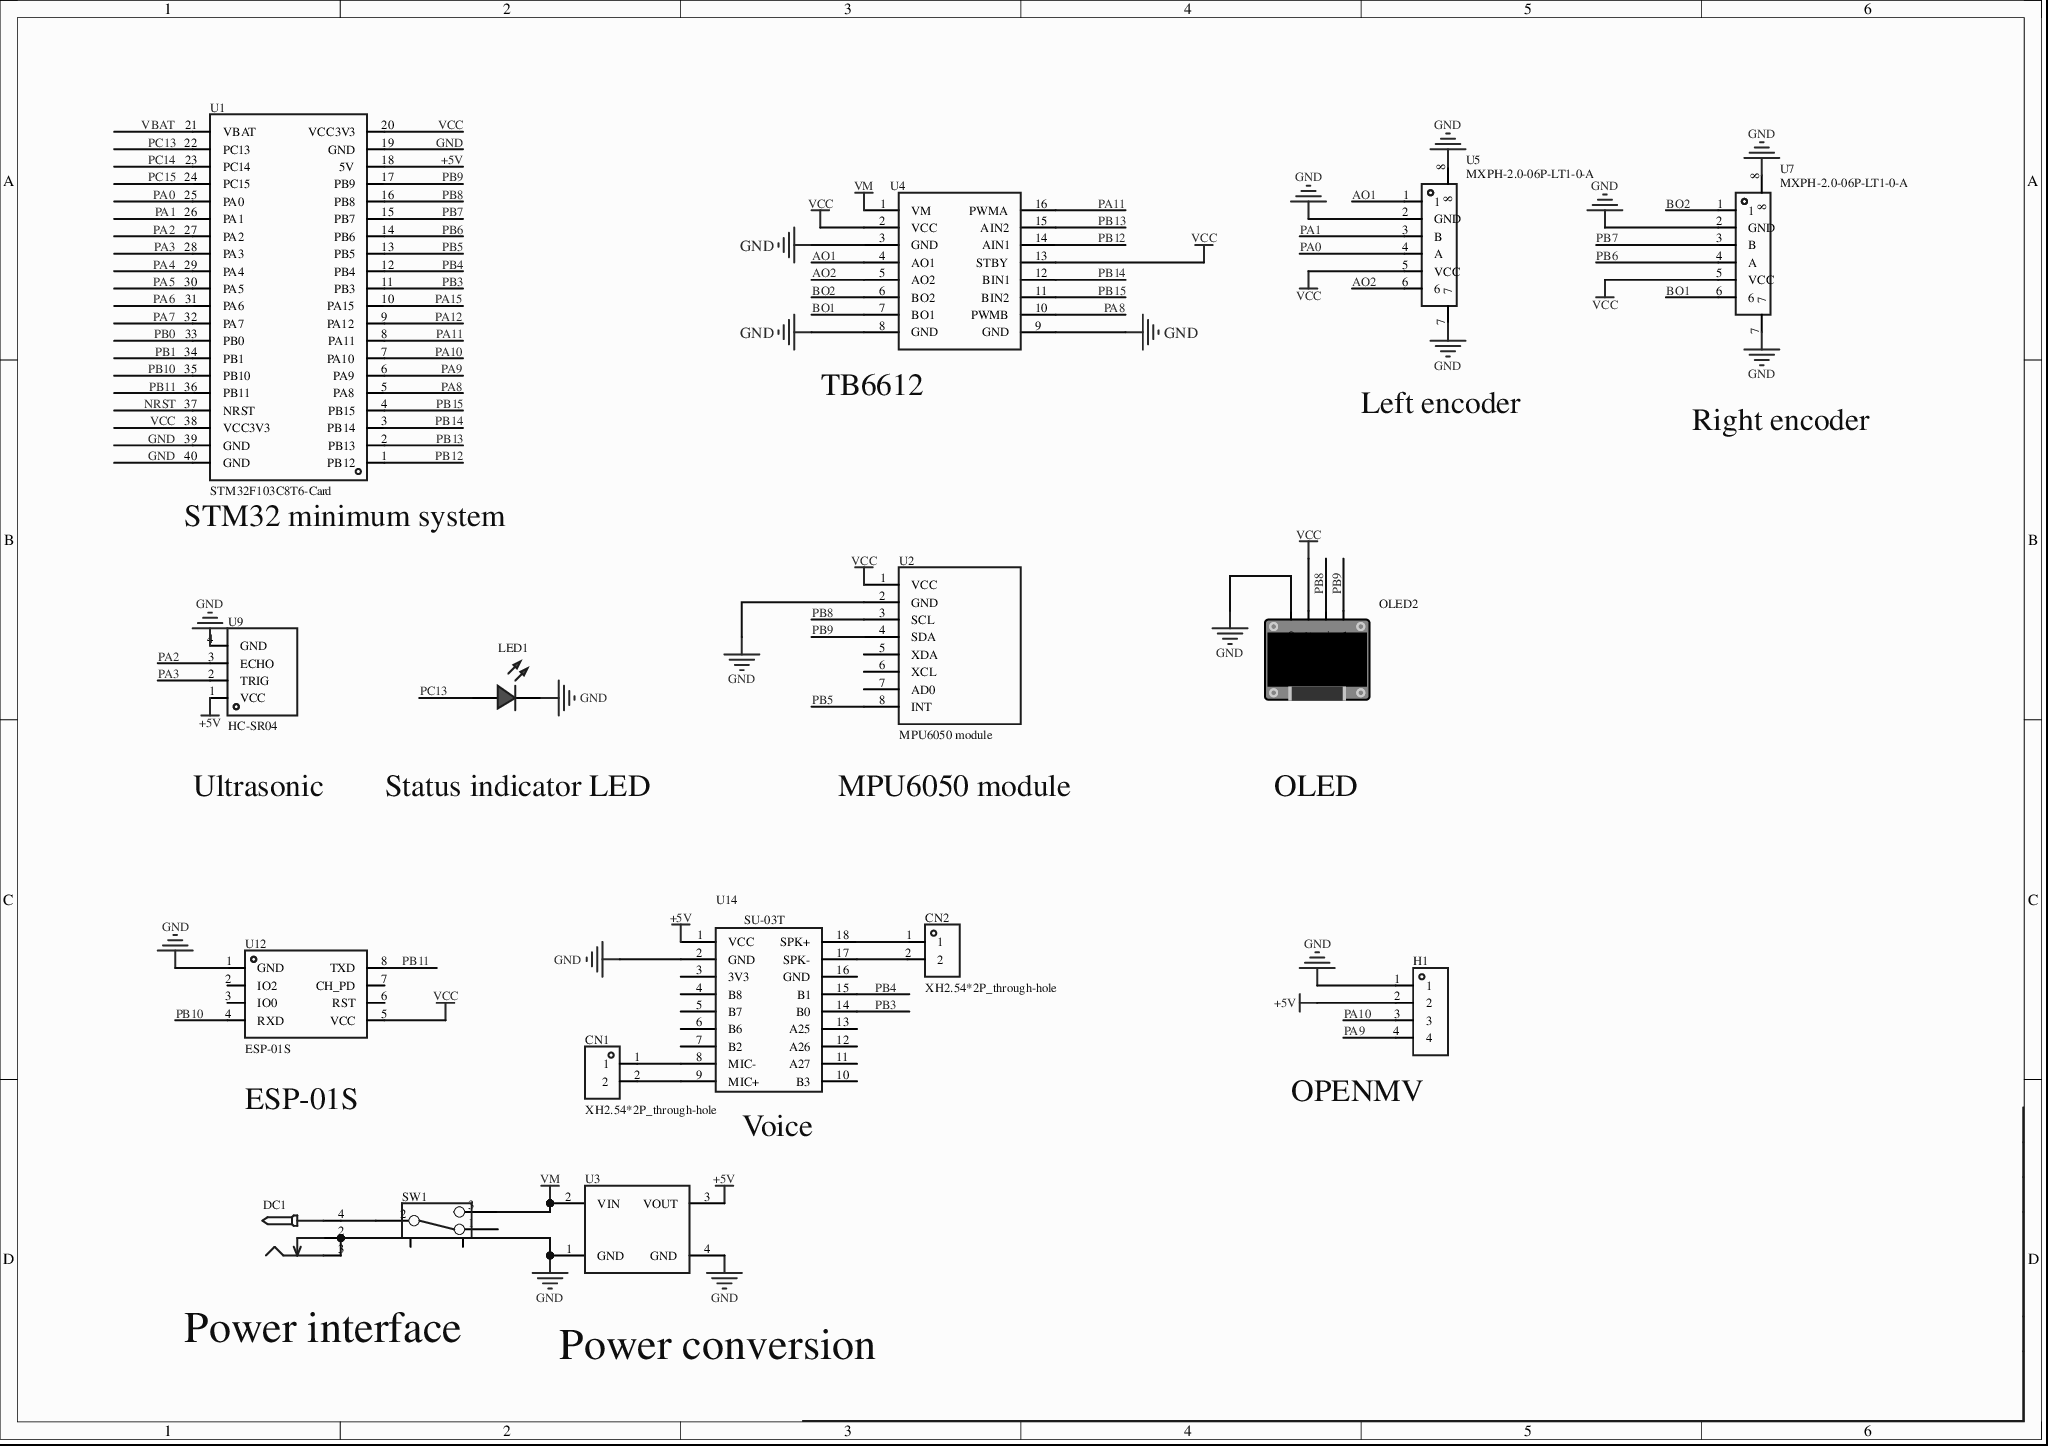
[diagram p0: MISC61229-3.schdoc]
# Altium project MISC61229-2.PrjPcb
1 sheet, 16 parts. Net scope: global (net labels, ports and power ports of the same name join across sheets).
Board file: MISC61229.pcbdoc

## Sheet MISC61229-3.schdoc
size 297 x 209 mm; Version: V1.0; @Project Name: MISC61229; @Page Count: 1; @Update Date: 2026-05-19; @Create Date: 2026-05-19; @Schematic Name: MISC61229; @Page No: 1; @Create Time: 23:22:16; @Update Time: 17:32:40; @Board Name: MISC61229

### Parts
CN1  XH2.54*2P_through-hole  [CONN-TH_2P-P2.50-XH2.54-2P]
CN2  XH2.54*2P_through-hole  [CONN-TH_2P-P2.50-XH2.54-2P]
DC1  (no value)  [DC-2.0]
H1  (no value)  [HDR-TH_4P-P2.54-V-M]
LED1  (no value)  [LED_TH-3mm]
OLED2  (no value)  [0.96OLED_4P]
SW1  (no value)  [拨动开关]
U1  STM32F103C8T6-Card  [CONN-TH_L53.3-W22.9_STM32F103C8T6-CARD]
U2  MPU6050 module  [MPU6050]
U3  (no value)  [MP1584主控]
U4  (no value)  [tb6612]
U5  MXPH-2.0-06P-LT1-0-A  [CONN-SMD_6P-P2.00_MXPH-2.0-6P-LT1-0-A]
U7  MXPH-2.0-06P-LT1-0-A  [CONN-SMD_6P-P2.00_MXPH-2.0-6P-LT1-0-A]
U9  HC-SR04  [TH_HC-SR04V]
U12  ESP-01S  [WIFIM-TH_ESP-01S]
U14  (no value)  [SU-03T]

### Nets
+5V: H1.2 U1.18(5V) U3.3(VOUT) U9.1(VCC) U14.1(VCC)
GND: DC1.2 DC1.3 H1.1 LED1.2(A) OLED2.1(GND) U1.19(GND) U1.39(GND) U1.40(GND) U2.2(GND) U3.1(GND) U3.4(GND) U4.3(GND) U4.8(GND) U4.9(GND) U5.2(GND) U5.7 U5.8 U7.2(GND) U7.7 U7.8 U9.4(GND) U12.1(GND) U14.2(GND)
VCC: OLED2.2(VCC) U1.20(VCC3V3) U1.38(VCC3V3) U2.1(VCC) U4.2(VCC) U4.13(STBY) U5.5(VCC) U7.5(VCC) U12.5(VCC)
VM: SW1.3 U3.2(VIN) U4.1(VM)
AO1: U4.4(AO1) U5.1
AO2: U4.5(AO2) U5.6
BO1: U4.7(BO1) U7.6
BO2: U4.6(BO2) U7.1
NRST: U1.37(NRST)
PA0: U1.25(PA0) U5.4(A)
PA1: U1.26(PA1) U5.3(B)
PA2: U1.27(PA2) U9.3(ECHO)
PA3: U1.28(PA3) U9.2(TRIG)
PA4: U1.29(PA4)
PA5: U1.30(PA5)
PA6: U1.31(PA6)
PA7: U1.32(PA7)
PA8: U1.5(PA8) U4.10(PWMB)
PA9: H1.4 U1.6(PA9)
PA10: H1.3 U1.7(PA10)
PA11: U1.8(PA11) U4.16(PWMA)
PA12: U1.9(PA12)
PA15: U1.10(PA15)
PB0: U1.33(PB0)
PB1: U1.34(PB1)
PB3: U1.11(PB3) U14.14(B0)
PB4: U1.12(PB4) U14.15(B1)
PB5: U1.13(PB5) U2.8(INT)
PB6: U1.14(PB6) U7.4(A)
PB7: U1.15(PB7) U7.3(B)
PB8: OLED2.3(SCL) U1.16(PB8) U2.3(SCL)
PB9: OLED2.4(SDA) U1.17(PB9) U2.4(SDA)
PB10: U1.35(PB10) U12.4(RXD)
PB11: U1.36(PB11) U12.8(TXD)
PB12: U1.1(PB12) U4.14(AIN1)
PB13: U1.2(PB13) U4.15(AIN2)
PB14: U1.3(PB14) U4.12(BIN1)
PB15: U1.4(PB15) U4.11(BIN2)
PC13: LED1.1(C) U1.22(PC13)
PC14: U1.23(PC14)
PC15: U1.24(PC15)
VBAT: U1.21(VBAT)
NetCN1_1: CN1.1 U14.8(MIC-)
NetCN1_2: CN1.2 U14.9(MIC+)
NetCN2_1: CN2.1 U14.18(SPK+)
NetCN2_2: CN2.2 U14.17(SPK-)
NetDC1_4: DC1.4 SW1.2

Not connected (* = marked no-connect by the designer): SW1 1 4 5; U2 5(XDA) 6(XCL) 7(AD0); U12 2(IO2)* 3(IO0)* 6(RST)* 7(CH_PD)*; U14 3(3V3) 4(B8) 5(B7) 6(B6) 7(B2) 10(B3) 11(A27) 12(A26) 13(A25) 16(GND)

### Notes on the sheet
- (near U4) TB6612
- Left encoder
- Right encoder
- (near U1) STM32 minimum system
- Ultrasonic
- Status indicator LED
- (near U2) MPU6050 module
- OLED
- (near U12) ESP-01S
- (near H1) OPENMV
- (near U14) Voice
- Power interface
- (near U3) Power conversion

### Library data of the parts
CN1 CN2 = XH2.54*2P_直插: AddInBom: yes; ModelId: 325c595e30db4df8abe76612dd40b0fa0819f05c4eef4c71ace90d822a990e87; ModelTransform: 295.275,228.346,0,180,0,0,-0.002,-20.079,-137.795; Symbol: XH2.54*2P_through-hole; Device: XH2.54*2P_through-hole; LCSC Part Name: XH2.54*2P_直插; SupplierPart: C9900008615; ManufacturerPart: XH2.54*2P_直插; Supplier Footprint: XH2.54_2P; JLCPCB Part Class: Extended Part; Supplier: LCSC; ConvertToPcb: yes; FootprintName: CONN-TH_2P-P2.50-XH2.54-2P; ModelName: CONN-TH_2P-P2.50-XH2.54-2P
DC1 = DC-005_2.0: Symbol: DC power connector; ConvertToPcb: yes; ModelId: f5f20b8a2308479b936ba3c2698865bb0819f05c4eef4c71ace90d822a990e87; ModelName: DC-IN-TH_DC-5520-1; ModelTransform: 372.05,551.18,582.68,90,0,0,137.8,0,-149.61; Device: DC-005_2.0; AddInBom: yes; Supplier Footprint: 插件; FootprintName: DC-2.0
H1 = HDR-M_2.54_1x4P: Symbol: PZ254V-11-04P; ConvertToPcb: yes; ModelId: 112f4d05e8d64e99ab9a333894bea4f90819f05c4eef4c71ace90d822a990e87; ModelName: HDR-TH_4P-P2.54-M-LI-1X4P; ModelTransform: 399.999,104.7242,0,0,0,0,0,0,-118.11; Device: HDR-M_2.54_1x4P; AddInBom: yes; SupplierPart: C492403; Supplier Footprint: 插件; FootprintName: HDR-TH_4P-P2.54-V-M
LED1 = LED_TH-R_3mm: ConvertToPcb: yes; ModelId: a497c992633541038a38947cdc58012f0819f05c4eef4c71ace90d822a990e87; ModelName: LED-TH-3mm_R; ModelTransform: 141.274,153.327,0,0,0,0,-5.984,0,-137.795; Symbol: LED_TH-R; Device: LED_TH-R_3mm; AddInBom: yes; FootprintName: LED_TH-3mm; Supplier Footprint: 插件
OLED2 = 0.96OLED模块_4P: Symbol: 0.96OLED module_4P; 3D Model: 79c000fdb68d45a296c2e9bedf4f9055; 3D Model Transform: 1393.69792,1318.895,0,0,0,0,0,-560.079,-137.795; ConvertToPcb: yes; Device: 0.96OLED module_4P; Supplier Footprint: 插件; AddInBom: yes; FootprintName: 0.96OLED_4P; ModelName: 0.96OLED_4P
SW1 = 拨动开关_正: Symbol: Toggle switch; Device: Toggle switch_positive; ConvertToPcb: yes; ModelId: 4321fe59a4074cbfb4989553f297c68f0819f05c4eef4c71ace90d822a990e87; ModelName: SW-TH_SS-12D02-VG4; ModelTransform: 370.09,208.7,472.35,0,0,0,0,0,-110; AddInBom: yes; Supplier Footprint: 插件; FootprintName: Toggle switch
U1 = STM32F103C8T6-Card: AddInBom: yes; Device: STM32F103C8T6-Card; Symbol: STM32F103C8T6-CARD; FootprintName: CONN-TH_L53.3-W22.9_STM32F103C8T6-CARD; LCSC Part Name: STM32F103C8T6-Card; SupplierPart: C9900077949; ManufacturerPart: STM32F103C8T6-Card; Supplier Footprint: 插件; Supplier: LCSC; ConvertToPcb: yes
U2 = MPU6050模块: AddInBom: yes; Symbol: MPU6050 module; Device: MPU6050 module; Value: MPU6050模块; ConvertToPcb: yes; FootprintName: MPU6050
U3 = MP1584: Adjustable output voltage, max 3A current; AddInBom: yes; Symbol: MP1584; Device: MP1584; ConvertToPcb: yes; FootprintName: MP1584 main controller
U4 = tb6612: AddInBom: yes; Symbol: tb6612; Device: tb6612; JLCPCB Part Class: Extended library; ConvertToPcb: yes; FootprintName: tb6612
U5 = MXPH-2.0-06P-LT1-0-A: Pin structure:1x6P;pitch:2mm;mounting:vertical SMD;series:PH;total pins:6P;rows:1;pins per row:6;rated current:2A;contact material:copper alloy;contact plating:tin;operating temperature:-25℃~+85℃;; Manufacturer: MAX(迈旭); Symbol: MXPH-2.0-06P-LT1-0-A_1; AddInBom: yes; ModelId: 7656877d212b4dcda05e79af15a508d50819f05c4eef4c71ace90d822a990e87; ModelTransform: 629.92,281.4955,0,180,0,0,0,26.22,0; Pins Structure: 1x6P; Pitch: 2mm; Reference Series: PH; Number of PINs Per Row: 6; Current Rating: 2A; Voltage Rating: 250V; Plastic Material: LCP; Flame Retardant Rating: UL94V-0; Device: MXPH-2.0-06P-LT1-0-A; LCSC Part Name: 象牙白 1x6P 间距:2mm 立贴 系列:PH; SupplierPart: C7542145; ManufacturerPart: MXPH-2.0-06P-LT1-0-A; Supplier Footprint: SMD,P=2mm; JLCPCB Part Class: Extended Part; Datasheet: https://item.szlcsc.com/datasheet/MXPH-2.0-06P-LT1-0-A/8645846.html; Supplier: LCSC; ConvertToPcb: yes; FootprintName: CONN-SMD_6P-P2.00_MXPH-2.0-6P-LT1-0-A; ModelName: CONN-SMD_6P-P2.00_MXPH-2.0-6P-LT1-0-A; Mounting Type: Vertical SMD; Number of Pins: 6P; Number of Rows: 1; Contact Material: Copper alloy; Contact Plating: Tin; Operating Temperature: -25℃~+85℃; Color: -
U7 = MXPH-2.0-06P-LT1-0-A: Pin structure:1x6P;pitch:2mm;mounting:vertical SMD;series:PH;total pins:6P;rows:1;pins per row:6;rated current:2A;contact material:copper alloy;contact plating:tin;operating temperature:-25℃~+85℃;; Manufacturer: MAX(迈旭); Symbol: MXPH-2.0-06P-LT1-0-A_1; 3D Model: 7656877d212b4dcda05e79af15a508d50819f05c4eef4c71ace90d822a990e87; 3D Model Transform: 629.92,281.4955,0,180,0,0,0,26.22,0; Pins Structure: 1x6P; Pitch: 2mm; Reference Series: PH; Number of PINs Per Row: 6; Current Rating: 2A; Voltage Rating: 250V; Plastic Material: LCP; Flame Retardant Rating: UL94V-0; AddInBom: yes; Device: MXPH-2.0-06P-LT1-0-A; LCSC Part Name: 象牙白 1x6P 间距:2mm 立贴 系列:PH; Supplier Part: C7542145; Manufacturer Part: MXPH-2.0-06P-LT1-0-A; Supplier Footprint: SMD,P=2mm; JLCPCB Part Class: Extended Part; Datasheet: https://item.szlcsc.com/datasheet/MXPH-2.0-06P-LT1-0-A/8645846.html; Supplier: LCSC; Mounting Type: Vertical SMD; Number of Pins: 6P; Number of Rows: 1; Contact Material: Copper alloy; Contact Plating: Tin; Operating Temperature: -25℃~+85℃; Color: -; ConvertToPcb: yes; FootprintName: CONN-SMD_6P-P2.00_MXPH-2.0-6P-LT1-0-A; ModelName: CONN-SMD_6P-P2.00_MXPH-2.0-6P-LT1-0-A
U9 = HC-SR04: Manufacturer: Universal Microelectronics; AddInBom: yes; Symbol: HC-SR04; Device: HC-SR04; LCSC Part Name: HC-SR04; Supplier Part: C19857336; Manufacturer Part: HC-SR04; Supplier Footprint: -; JLCPCB Part Class: Extended library; Datasheet: https://atta.szlcsc.com/upload/public/pdf/source/20240122/47B8E374E428935B7962A2189EF91AAC.pdf; Supplier: LCSC; ConvertToPcb: yes; FootprintName: TH_HC-SR04V
U12 = ESP-01S_C111009: 3D Model: eb7175da78ae48b3b1568cfe3027405f0819f05c4eef4c71ace90d822a990e87; 3D Model Transform: 582.676,976.37608,0,0,0,0,0,388.346,-118.11; AddInBom: yes; Symbol: ESP-01S; Device: ESP-01S_C111009; LCSC Part Name: ESP-01S; Supplier Part: C111009; Manufacturer Part: ESP-01S; Supplier Footprint: -; JLCPCB Part Class: Extended Part; Supplier: LCSC; ConvertToPcb: yes; FootprintName: WIFIM-TH_ESP-01S; ModelName: WIFIM-TH_ESP-01S
U14 = SU-03T: AddInBom: yes; Symbol: SU-03T; Device: SU-03T; ConvertToPcb: yes; FootprintName: SU-03T